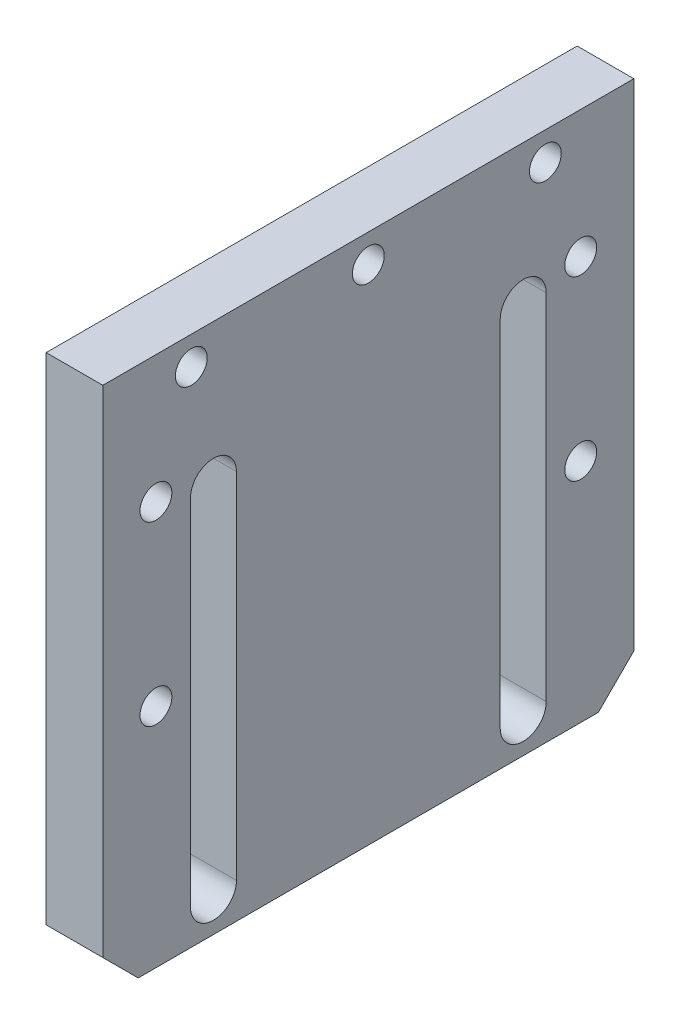
SolidWorks part; units mm, degrees
ref_plane "前视基准面" through (0, 0, 0) normal (0, 0, 1) x (1, 0, 0)
ref_plane "上视基准面" through (0, 0, 0) normal (0, 1, 0) x (1, 0, 0)
ref_plane "右视基准面" through (0, 0, 0) normal (1, 0, 0) x (0, 0, -1)
sketch "草图1" plane through (0, 0, 0) normal (1, 0, 0) x (0, 0, -1)
  line L1 (-75, 75) -> (75, 75)
  line L2 (-75, 75) -> (-75, -75)
  line L3 (-75, -75) -> (75, -75)
  line L4 (75, 75) -> (75, -75)
  line L5 (-75, 75) -> (75, -75) construction
  line L6 (-75, -75) -> (75, 75) construction
  point P0 (0, 0)
  dimension "D1" = 150
  dimension "D2" = 150
extrude "凸台-拉伸1" add sketch "草图1" along normal blind 16
sketch "草图3" plane through (16, 0, 0) normal (1, 0, 0) x (0, 0, -1)
  line L0 (-43.7534, 35) -> (-43.7534, -65) construction
  line L1 (-37.2534, 35) -> (-37.2534, -65)
  line L2 (-50.2534, 35) -> (-50.2534, -65)
  line L3 (43.7534, 35) -> (43.7534, -65) construction
  line L4 (50.2534, 35) -> (50.2534, -65)
  line L5 (37.2534, 35) -> (37.2534, -65)
  line L6 (0, 0) -> (0, 108.9704) construction
  line L7 (-75, -75) -> (75, -75) construction
  arc A0 (-37.2534, 35) -> (-50.2534, 35) centre (-43.7534, 35) ccw
  arc A1 (-50.2534, -65) -> (-37.2534, -65) centre (-43.7534, -65) ccw
  arc A2 (50.2534, 35) -> (37.2534, 35) centre (43.7534, 35) ccw
  arc A3 (37.2534, -65) -> (50.2534, -65) centre (43.7534, -65) ccw
  point P2 (-43.7534, -15)
  point P7 (43.7534, -15)
  dimension "D1" = 60
  dimension "D2" = 100
  dimension "D3" = 13
extrude "切除-拉伸1" cut sketch "草图3" against normal through all
hole_wizard "打孔尺寸(%根据)内六角圆柱头螺钉的类型1" positions "草图4" profile "草图5" counterbore size "M8" standard "GB"
sketch "草图4" plane through (0, 0, 0) normal (-1, 0, 0) x (0, 0, 1)
  line L0 (0, 0) -> (0, 99.4814) construction
  line L2 (-75, 75) -> (75, 75) construction
  point P0 (-50, 67)
  point P2 (0, 67)
  point P4 (50, 67)
  dimension "D1" = 8
  dimension "D2" = 100
sketch "草图5" plane through (0, 67, -50) normal (0, 1, 0) x (0, 0, 1)
  line L0 (0, 0) -> (0, 31.9539)
  line L1 (0, 31.9539) -> (4.5, 29.25)
  line L2 (4.5, 29.25) -> (4.5, 9)
  line L3 (4.5, 9) -> (7.5, 9)
  line L4 (7.5, 9) -> (7.5, 0)
  line L5 (7.5, 0) -> (0, 0)
  line L10 (0, 31.9539) -> (-4.5, 29.25) construction
  line L11 (0, -6.35) -> (0, 107.95) construction
  dimension "孔直径" = 9
  dimension "孔深度" = 29.25
  dimension "柱形沉头孔直径" = 15
  dimension "柱形沉头孔深度" = 9
  dimension "导头角度" = 118
hole_wizard "打孔尺寸(%根据)内六角圆柱头螺钉的类型2" positions "草图6" profile "草图7" counterbore size "M8" standard "GB"
sketch "草图6" plane through (0, 0, 0) normal (-1, 0, 0) x (0, 0, 1)
  line L0 (0, 0) -> (0, 52.8466) construction
  line L2 (-75, -75) -> (-75, 75) construction
  line L3 (-75, 75) -> (75, 75) construction
  point P0 (-60, 39)
  point P2 (-60, -11)
  point P4 (60, 39)
  point P6 (60, -11)
  dimension "D1" = 15
  dimension "D2" = 50
  dimension "D3" = 36
sketch "草图7" plane through (0, 39, -60) normal (0, 1, 0) x (0, 0, 1)
  line L0 (0, 0) -> (0, 31.9539)
  line L1 (0, 31.9539) -> (4.5, 29.25)
  line L2 (4.5, 29.25) -> (4.5, 9)
  line L3 (4.5, 9) -> (7.5, 9)
  line L4 (7.5, 9) -> (7.5, 0)
  line L5 (7.5, 0) -> (0, 0)
  line L10 (0, 31.9539) -> (-4.5, 29.25) construction
  line L11 (0, -6.35) -> (0, 107.95) construction
  dimension "孔直径" = 9
  dimension "孔深度" = 29.25
  dimension "柱形沉头孔直径" = 15
  dimension "柱形沉头孔深度" = 9
  dimension "导头角度" = 118
chamfer "倒角1" distance 10 angle 45 2 edges at (8, -75, 75) (8, -75, -75)
